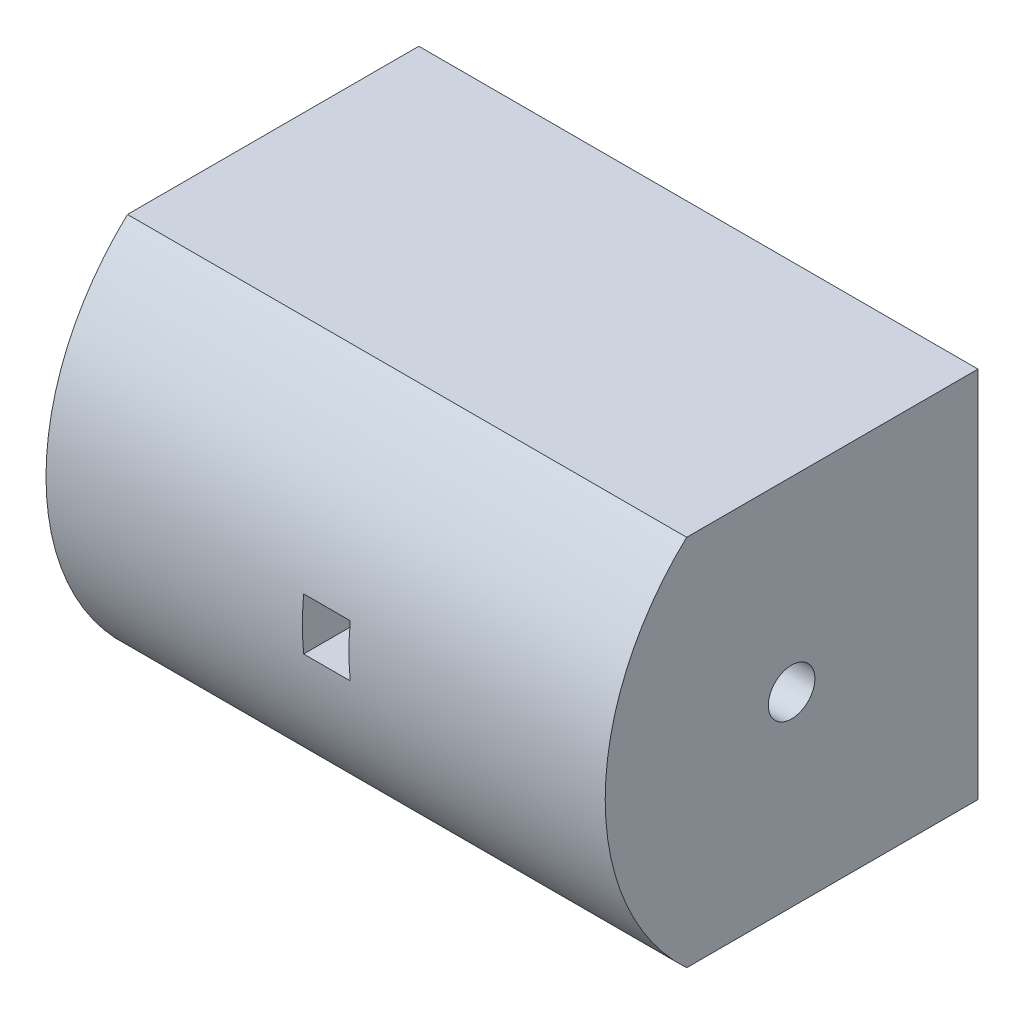
SolidWorks part; units mm, degrees
material "Zoltek Panex 33"
ref_plane "前视基准面" through (0, 0, 0) normal (0, 0, 1) x (1, 0, 0)
ref_plane "上视基准面" through (0, 0, 0) normal (0, 1, 0) x (1, 0, 0)
ref_plane "右视基准面" through (0, 0, 0) normal (1, 0, 0) x (0, 0, -1)
other "Configuration Table"
sketch "草图1" plane through (0, 0, 0) normal (0, 0, 1) x (1, 0, 0)
  line L1 (-60, -40) -> (60, -40)
  line L2 (-60, -40) -> (-60, 40)
  line L3 (-60, 40) -> (60, 40)
  line L4 (60, -40) -> (60, 40)
  line L5 (-60, -40) -> (60, 40) construction
  line L6 (-60, 40) -> (60, -40) construction
  point P0 (0, 0)
  dimension "D1" = 120
  dimension "D2" = 80
extrude "凸台-拉伸1" add sketch "草图1" along normal blind 80
sketch "草图2" plane through (-60, 0, 0) normal (-1, 0, 0) x (0, 0, 1)
  circle A0 centre (40, 0) radius 5
  dimension "D1" = 10
extrude "切除-拉伸1" cut sketch "草图2" against normal through all
sketch "草图4" plane through (60, 0, 0) normal (1, 0, 0) x (0, 0, -1)
  line L2 (-62.5169, 40) -> (-80, 40)
  line L3 (-80, 40) -> (0, 40) construction
  line L5 (-80, -40) -> (0, -40) construction
  line L10 (-80, 40) -> (-80, -40)
  line L11 (-80, -40) -> (-62.5169, -40)
  arc A1 (-62.5169, 40) -> (-62.5169, -40) centre (-25.5, 0) ccw
  line M8 (0, 40) -> (-80, 40)
  line M9 (-80, 40) -> (-80, -40)
  line M10 (-80, -40) -> (0, -40)
extrude "切除-拉伸2" cut sketch "草图4" against normal through all contours A1 M8 M9 | A1 L10 M10
sketch "草图5" plane through (0, 0, 0) normal (0, 0, -1) x (-1, 0, 0)
  line L1 (-5, -5.59) -> (5, -5.59)
  line L2 (-5, -5.59) -> (-5, 5.59)
  line L3 (-5, 5.59) -> (5, 5.59)
  line L4 (5, -5.59) -> (5, 5.59)
  line L5 (-5, -5.59) -> (5, 5.59) construction
  line L6 (-5, 5.59) -> (5, -5.59) construction
  point P0 (0, 0)
  dimension "D1" = 10
  dimension "D2" = 11.18
extrude "切除-拉伸3" cut sketch "草图5" against normal up to next
sketch "草图6" plane through (0, 0, 0) normal (0, 0, -1) x (-1, 0, 0)
  line L1 (-5, -5.59) -> (5, -5.59)
  line L2 (-5, -5.59) -> (-5, 5.59)
  line L3 (-5, 5.59) -> (5, 5.59)
  line L4 (5, -5.59) -> (5, 5.59)
  line L5 (-5, -5.59) -> (5, 5.59) construction
  line L6 (-5, 5.59) -> (5, -5.59) construction
  point P0 (0, 0)
extrude "凸台-拉伸2" add sketch "草图6" against normal blind 50
